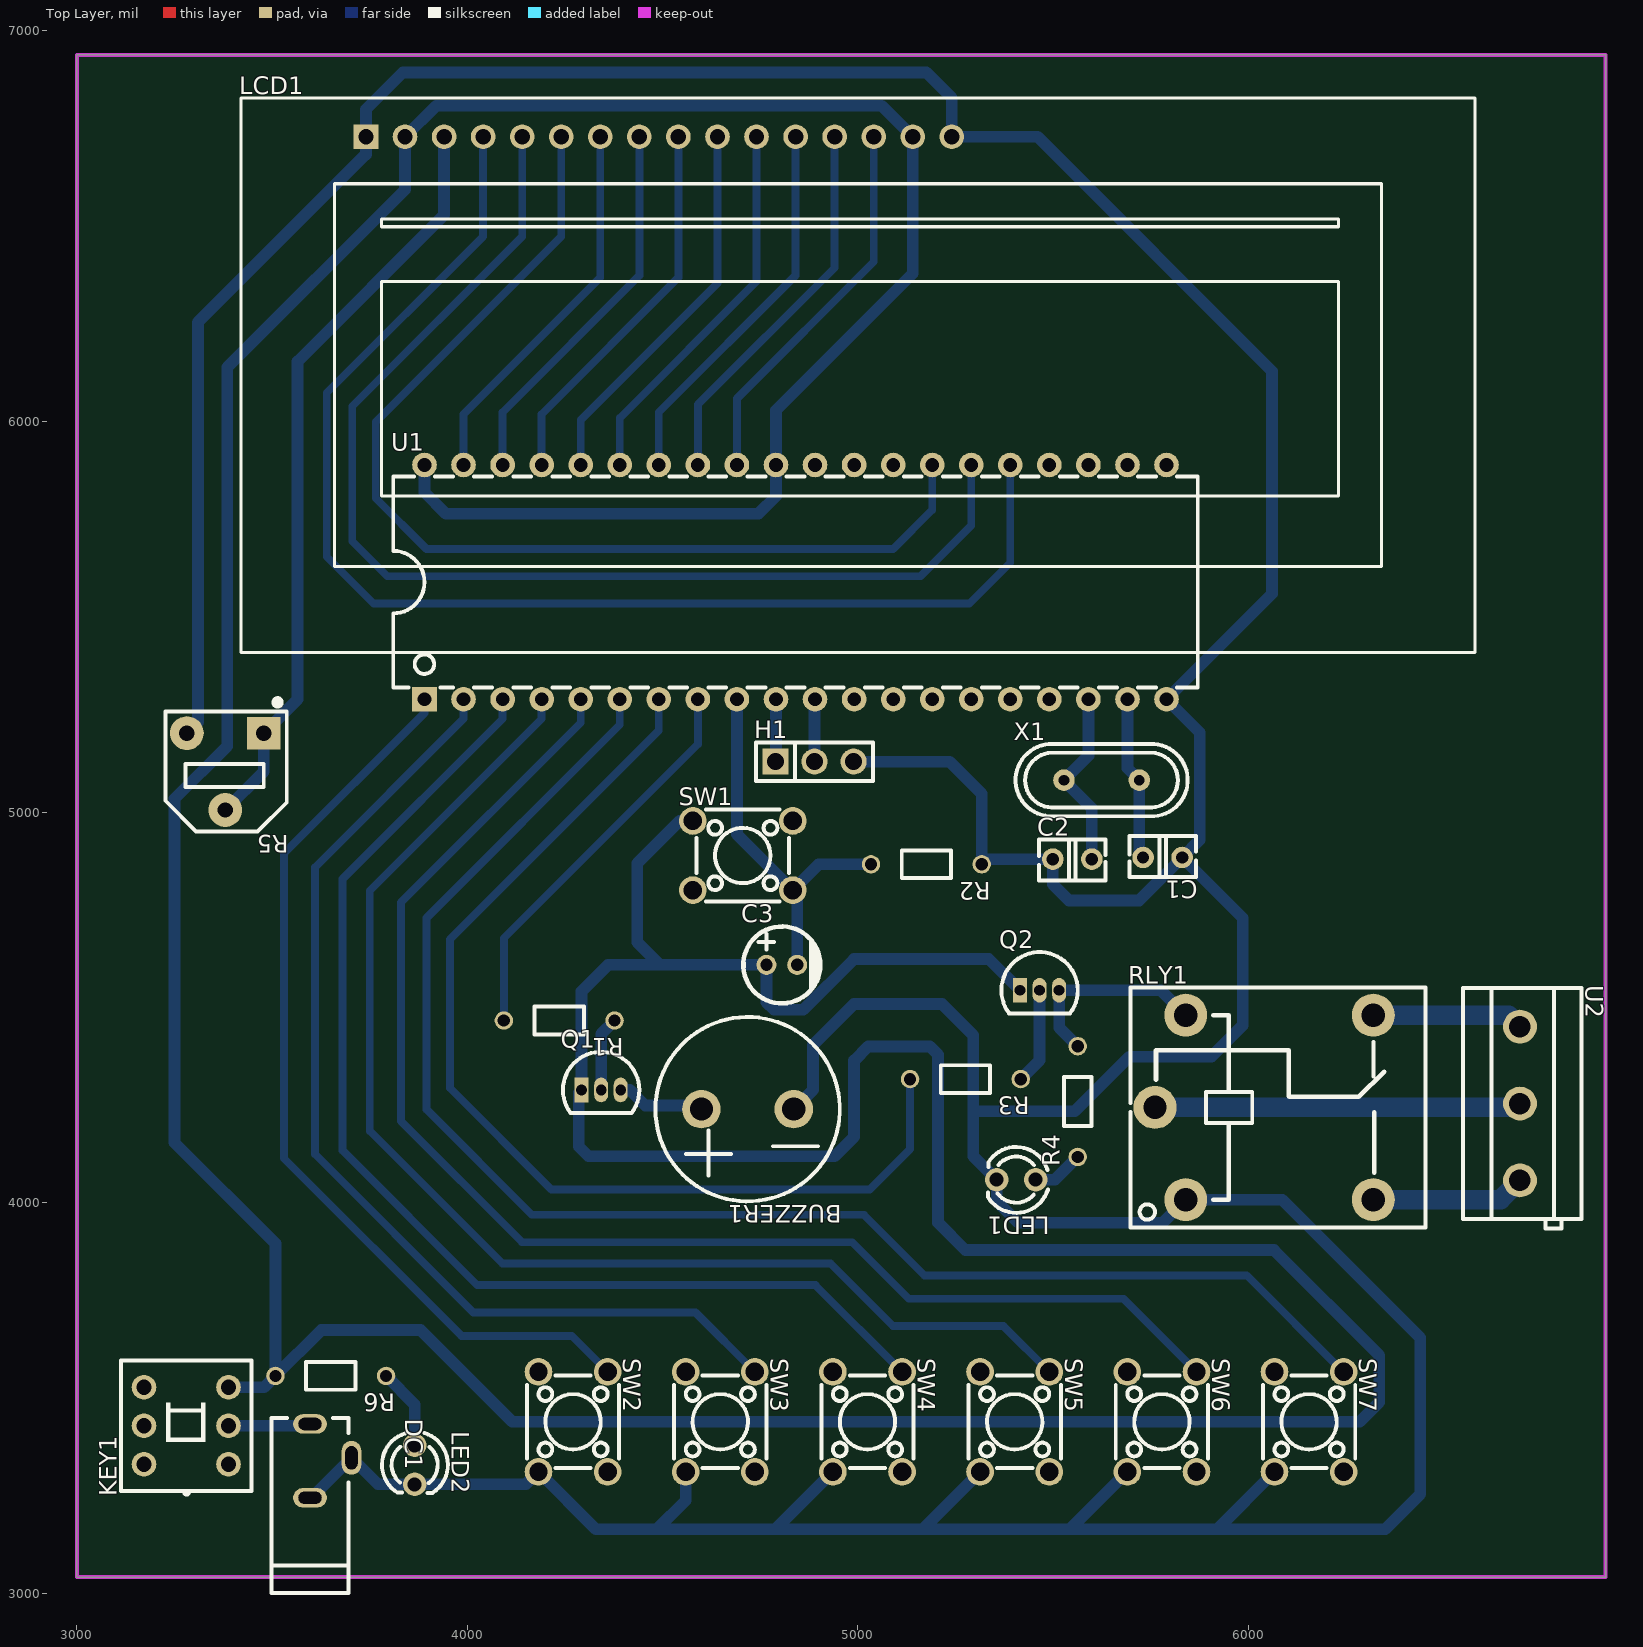
[diagram p0: Top Layer view]
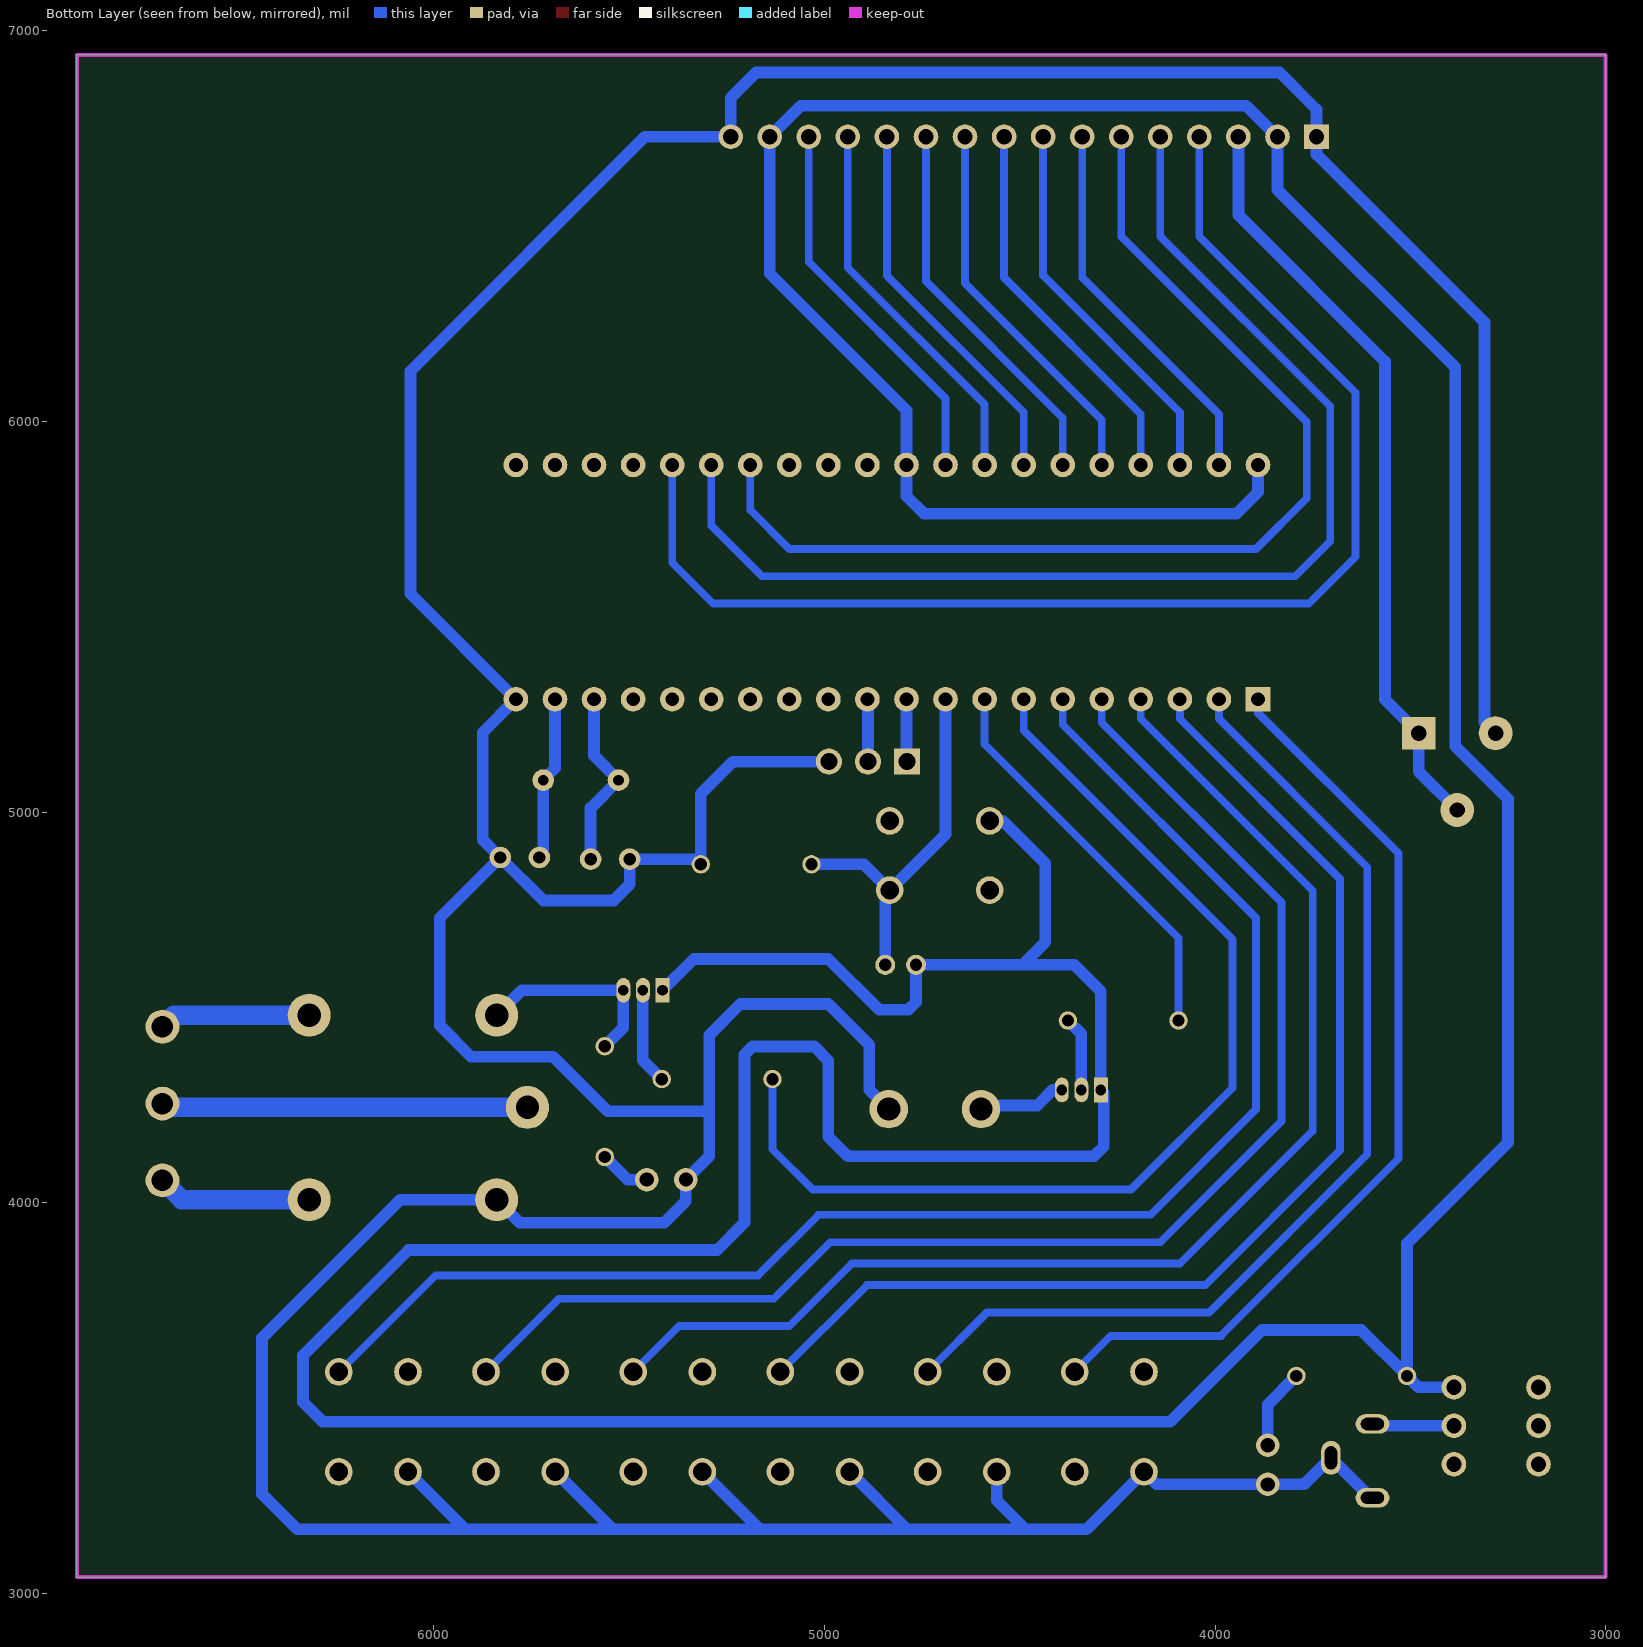
[diagram p1: Bottom Layer view, seen from below]
# Altium PCB MISC50235.pcbdoc
Units mil, origin at the board's own origin, x right, y up, seen from the top; angles counter-clockwise.
Board outline 3914.17 x 3897.64 mil, 2 copper layers (Top Layer, Bottom Layer), stack 62.206 mil thick; 29 components, 48 nets, 137 pads, 0 vias.

## Layer stack, top to bottom
Top Solder Mask Layer: solder mask 0.394, Dk 3.3
Top Layer: signal copper 1.379
Dielectric1: surface 59.449, FR4, Dk 4.5
Bottom Layer: signal copper 1.378
Bottom Solder Mask Layer: solder mask 0.394, Dk 3.3

## Board outline
3000,6938.58 3000,3040.95 6914.17,3040.95 6914.17,6938.58

## Design rules (kind name [scope] priority, off if disabled: settings)
BoardOutlineClearance copperThickness2oz_1 [All] p2 off: genericclearance=7.99 ignorepadtopadclearanceinfootprint=FALSE except(0: Arc-SplitContinuation Track-SplitContinuation SMDPad-SplitContinuation THPad-SplitContinuation Via-SplitContinuation Fill-SplitContinuation Region-SplitContinuation Poly-SplitContinuation Text-SplitContinuation Hole-SplitContinuation; 5.98: Arc-CutoutEdge SMDPad-CutoutEdge THPad-CutoutEdge Via-CutoutEdge Fill-CutoutEdge Region-CutoutEdge Text-CutoutEdge; 6.93: Hole-OutlineEdge Hole-CutoutEdge; 10: Poly-OutlineEdge Poly-CutoutEdge; 11.81: Arc-OutlineEdge Track-OutlineEdge SMDPad-OutlineEdge THPad-OutlineEdge Via-OutlineEdge Fill-OutlineEdge Region-OutlineEdge Text-OutlineEdge Track-CutoutEdge)
BoardOutlineClearance copperThickness1oz_1 [All] p4: genericclearance=4.02 ignorepadtopadclearanceinfootprint=FALSE except(0: Arc-SplitContinuation Track-SplitContinuation SMDPad-SplitContinuation THPad-SplitContinuation Via-SplitContinuation Fill-SplitContinuation Region-SplitContinuation Poly-SplitContinuation Text-SplitContinuation Hole-SplitContinuation; 6: SMDPad-CutoutEdge THPad-CutoutEdge Via-CutoutEdge Fill-CutoutEdge Region-CutoutEdge Text-CutoutEdge; 6.93: Hole-OutlineEdge Hole-CutoutEdge; 10: Poly-OutlineEdge Poly-CutoutEdge; 11.8: Arc-OutlineEdge Track-OutlineEdge SMDPad-OutlineEdge THPad-OutlineEdge Via-OutlineEdge Fill-OutlineEdge Region-OutlineEdge Text-OutlineEdge; 11.81: Arc-CutoutEdge Track-CutoutEdge)
Clearance copperThickness2oz [All] p1 off: gap=7.99 ignorepadtopadclearanceinfootprint=FALSE except(5.98: SMDPad-Track SMDPad-SMDPad THPad-Track SMDPad-THPad THPad-THPad Track-Via SMDPad-Via THPad-Via Via-Via Fill-Track Region-Track Fill-SMDPad Region-SMDPad Fill-THPad Region-THPad Fill-Via Region-Via Fill-Fill Fill-Region Region-Region Arc-Track Arc-SMDPad Arc-THPad Arc-Via Fill-Arc Region-Arc Arc-Arc Text-Track SMDPad-Text Text-THPad Text-Via Fill-Text Region-Text Arc-Text Text-Text; 6.93: Hole-Track Hole-SMDPad Hole-THPad Hole-Via Fill-Hole Region-Hole Hole-Arc Hole-Text; 10: Poly-Track Poly-SMDPad Poly-THPad Poly-Via Poly-Fill Poly-Region Poly-Poly Poly-Arc Poly-Text Poly-Hole)
Clearance copperThickness1oz [All] p3: gap=4.02 ignorepadtopadclearanceinfootprint=FALSE except(5.98: SMDPad-Track SMDPad-SMDPad THPad-Track SMDPad-THPad THPad-THPad Track-Via SMDPad-Via THPad-Via Via-Via Fill-Track Region-Track Fill-SMDPad Region-SMDPad Fill-THPad Region-THPad Fill-Via Region-Via Fill-Fill Fill-Region Region-Region; 6: Arc-Track Arc-SMDPad Arc-THPad Arc-Via Fill-Arc Region-Arc Arc-Arc Text-Track SMDPad-Text Text-THPad Text-Via Fill-Text Region-Text Arc-Text Text-Text; 6.93: Hole-Track Hole-SMDPad Hole-THPad Hole-Via Fill-Hole Region-Hole Hole-Arc Hole-Text; 10: Poly-Track Poly-SMDPad Poly-THPad Poly-Via Poly-Fill Poly-Region Poly-Poly Poly-Arc Poly-Text Poly-Hole)
Creepage creepage [All] p1: checkdistance=0 ignoreinternallayers=TRUE applytopolygonpour=TRUE
DiffPairsRouting differentialPair [All] p1: maxlimit=6 minlimit=6 mostfreqgap=6 toplayer_minwidth=5 toplayer_prefwidth=10 toplayer_maxwidth=100 toplayer_mingap=6 toplayer_prefgap=6 toplayer_maxgap=6 bottomlayer_minwidth=5 bottomlayer_prefwidth=10 bottomlayer_maxwidth=100 bottomlayer_mingap=6 bottomlayer_prefgap=6 bottomlayer_maxgap=6 maxuncoupledlength=10
HoleToHoleClearance otherClearance [All] p1: gap=11.81 allowstackedmicrovias=TRUE
Length netLength [All] p1: minlimit=0 maxlimit=0
MatchedLengths netLengthTolerance [All] p1: tolerance=1000
PasteMaskExpansion pasteMaskExpansion [All] p1: expansion=0
PlaneConnect innerPlane [All] p1: planeconnectstyle=Relief reliefexpansion=20 reliefentries=4 reliefconductorwidth=10 reliefairgap=10
PolygonConnect copperRegion [All] p1: connectstyle=Relief reliefconductorwidth=10 reliefentries=4 polygonreliefangle="90 Angle" airgapwidth=10 via.connectstyle=Relief via.reliefconductorwidth=10 via.reliefentries=4 via.polygonreliefangle="90 Angle" via.airgapwidth=10
RoutingVias viaSize [All] p1: holewidth=12.01 width=24.02 viastyle="Through Hole" minholewidth=11.81 minwidth=19.68 maxholewidth=248.03 maxwidth=393.7
SolderMaskExpansion solderMaskExpansion [IsVia] p1: expansion=-1000 istentingtop=TRUE
SolderMaskExpansion solderMaskExpansion [All] p2: expansion=2 istentingtop=FALSE
Width copperThickness2oz_2 [All] p1 off: maxlimit=100 minlimit=8 preferedwidth=10
Width copperThickness1oz_2 [All] p2: maxlimit=100 minlimit=5 preferedwidth=10

## Components (designator, comment, footprint, x,y, rotation, side; value= is the part's Value field where it differs from the comment)
BUZZER1 "buzzer" BUZ-TH_BD12.0-P6.00-D0.9-RD 4717.32,4239.13 r180 top
C1 "30pF" CAP-TH_L3.8-W2.5-P2.54-D0.50 5780,4883.58 r180 top
C2 "30pF" CAP-TH_L3.8-W2.5-P2.54-D0.50 5548.8,4879.31 r0 top
C3 "10uF" CAP-TH_BD5.0-P2.00-D0.8-FD-10UF50VC110GL 4805,4608.58 r0 top
DC1 "DC-002" DC-IN-TH_DC-3510 3650,3338.58 r270 top
H1 "" HDR-TH_3P-P2.54-V-M 4888.8,5129.04 r0 top
KEY1 "无自锁开关 8.5×8.5 无声" SW-TH_6P-L8.5-W8.5-P2.54 3280,3428.58 r90 top
LCD1 "HS1602A" LCD1602 5000,6118.58 r0 top
LED1 "" LED_TH-3mm 5405,4058.58 r180 top
LED2 "" LED_TH-3mm 3865,3328.58 r270 top
Q1 "" S8550P_TO-92 4342.32,4288.34 r0 top
Q2 "" S8550P_TO-92 5465,4543.58 r0 top
R1 "1kΩ" Res_1/8W 4235,4468.58 r180 top
R2 "10kΩ" Res_1/8W 5175,4868.58 r180 top
R3 "1kΩ" Res_1/8W 5275,4318.58 r180 top
R4 "1kΩ" Res_1/8W 5565,4258.58 r90 top
R5 "10kΩ" RES-ADJ-SMD_RM065-V1 3380,5103.58 r180 top
R6 "1kΩ" Res_1/8W 3650,3558.58 r180 top
RLY1 "SRD-05VDC-SL-C" RELAY-TH_SRD-XXVDC-XL-C 6040,4243.58 r0 top
SW1 "" SW-TH_4P-L6.0-W6.0-P4.50-LS6.5 4705,4888.58 r0 top
SW2 "" SW-TH_4P-L6.0-W6.0-P4.50-LS6.5 4270.47,3438.58 r270 top
SW3 "" SW-TH_4P-L6.0-W6.0-P4.50-LS6.5 4647.38,3438.58 r270 top
SW4 "" SW-TH_4P-L6.0-W6.0-P4.50-LS6.5 5024.28,3438.58 r270 top
SW5 "" SW-TH_4P-L6.0-W6.0-P4.50-LS6.5 5401.19,3438.58 r270 top
SW6 "" SW-TH_4P-L6.0-W6.0-P4.50-LS6.5 5778.09,3438.58 r270 top
SW7 "" SW-TH_4P-L6.0-W6.0-P4.50-LS6.5 6155,3438.58 r270 top
U1 "STC89C52RC-40I-PDIP40" DIP-40_L52.0-W13.7-P2.54-LS15.2-BL 4840,5588.58 r0 top
U2 "KF301-5.0-3P" CONN-TH_3P-P5.00_KF301-5.0-3P 6695,4253.58 r270 top
X1 "11.0592MHz" OSC-TH_L11.1-W4.7-P4.88 5623.8,5081.61 r0 top

## Footprints (in the part's own frame and the unit in brackets; to place one, negate y for a bottom-side part, rotate by r counter-clockwise, add the part's x,y. Pads: shape width x height; smd on the part's side, far side on the other; paste and mask are expansions set on the pad)
BUZ-TH_BD12.0-P6.00-D0.9-RD [mm]
  round 2.5 hole 1.5 paste+0 mask+0.05: 1(-3,0) 2(3,0)
  silkscreen extent -5.99,-5.99 5.99,5.99
CAP-TH_BD5.0-P2.00-D0.8-FD-10UF50VC110GL [mm]
  round 1.3 hole 0.8: 1(-1,0) 2(1,0)
  silkscreen extent -2.5,-2.5 2.5,2.5
CAP-TH_L3.8-W2.5-P2.54-D0.50 [mm]
  round 1.4 hole 0.8 paste+0 mask+0.05: 1(-1.27,0) 2(1.27,0)
  silkscreen extent -2.16,-1.4 2.16,1.27
CONN-TH_3P-P5.00_KF301-5.0-3P [mm]
  round 2.2 hole 1.4: 1(-5,0) 2(0,0) 3(5,0)
  silkscreen extent -7.5,-3.7 8.13,4
DC-IN-TH_DC-3510 [mm]
  oval 1.27x2.2 hole 0.8 slot 1.5 at 90 deg: 1(-2.4,-1.35) 2(2.4,-1.35)
  oval 2.2x1.27 hole 0.8 slot 1.5 at 0 deg: 3(-0.2,1.35)
  silkscreen extent -2.8,-3.85 8.6,1.15
DIP-40_L52.0-W13.7-P2.54-LS15.2-BL [mil]
  rect 63x63 hole 35: 1(-950,-300)
  round 63 hole 35: 2(-850,-300) 3(-750,-300) 4(-650,-300) 5(-550,-300) 6(-450,-300) 7(-350,-300) 8(-250,-300) 9(-150,-300) 10(-50,-300) 11(50,-300) 12(150,-300) 13(250,-300) 14(350,-300) 15(450,-300) 16(550,-300) 17(650,-300) 18(750,-300) 19(850,-300) 20(950,-300) 21(950,300) 22(850,300) 23(750,300) 24(650,300) 25(550,300) 26(450,300) 27(350,300) 28(250,300) 29(150,300) 30(50,300) 31(-50,300) 32(-150,300) 33(-250,300) 34(-350,300) 35(-450,300) 36(-550,300) 37(-650,300) 38(-750,300) 39(-850,300) 40(-950,300)
  silkscreen extent -1030,-270 1030,270
HDR-TH_3P-P2.54-V-M [mm]
  rect 1.7x1.7 hole 1.1: 1(-2.54,0)
  round 1.7 hole 1.1: 2(0,0) 3(2.54,0)
  silkscreen extent -3.81,-1.25 3.81,1.25
LCD1602 [mm]
  rect 1.6x1.6 hole 1: 1(-32,15.5)
  round 1.6 hole 1: 2(-29.46,15.5) 3(-26.92,15.5) 4(-24.38,15.5) 5(-21.84,15.5) 6(-19.3,15.5) 7(-16.76,15.5) 8(-14.22,15.5) 9(-11.68,15.5) 10(-9.14,15.5) 11(-6.6,15.5) 12(-4.06,15.5) 13(-1.52,15.5) 14(1.02,15.5) 15(3.56,15.5) 16(6.1,15.5)
  silkscreen extent -40.13,-18.03 40.13,18.03
LED_TH-3mm [mil]
  round 60 hole 36 paste+0 mask+2: 1(-50,0) 2(50,0)
  silkscreen extent -81,-84 72,85
OSC-TH_L11.1-W4.7-P4.88 [mm]
  round 1.4 hole 0.7: 1(-2.45,0) 2(2.45,0)
  silkscreen extent -5.59,-2.35 5.6,2.35
RELAY-TH_SRD-XXVDC-XL-C [mil]
  round 110 hole 60: 1(-200.79,-236.22) 2(279.52,-236.2) 3(279.53,236.2) 4(-200.79,236.22) 5(-279.53,0)
  silkscreen extent -342,-307 413,307
RES-ADJ-SMD_RM065-V1 [mm]
  rect 2.2x2.1 hole 1 paste+0 mask+0.05: 1(-2.5,-2.5)
  round 2.2 hole 1 paste+0 mask+0.05: 2(0,2.5) 3(2.5,-2.5)
  silkscreen extent -4,-4.7 3.9,3.9
Res_1/8W [mil]
  round 47.2 hole 31.5 paste+0 mask+2: 1(-141.7,2.48) 2(141.7,2.48)
  silkscreen extent -63,-33 63,38
S8550P_TO-92 [mm]
  rect 0.9x1.6 hole 0.7 paste+0 mask+0.051: 1(-1.27,0)
  oval 0.9x1.6 hole 0.7 paste+0 mask+0.051: 2(0,0) 3(1.27,0)
  silkscreen extent -2.48,-1.5 2.48,2.48
SW-TH_4P-L6.0-W6.0-P4.50-LS6.5 [mm]
  round 1.8 hole 1.2: 1(-3.25,2.25) 2(3.25,2.25) 3(-3.25,-2.25) 4(3.25,-2.25)
  silkscreen extent -3,-3 3,3
SW-TH_6P-L8.5-W8.5-P2.54 [mm]
  round 1.6 hole 1: 1(-2.5,-2.75) 2(0,-2.75) 3(2.5,-2.75) 4(-2.5,2.75) 5(0,2.75) 6(2.5,2.75)
  silkscreen extent -4.47,-4.25 4.25,4.25

## Nets (pads, with @x,y where several pads share a name; then routed paths per layer and width w, separated by ;. In a path a pad name is that pad's centre, name@x,y a point inside that pad or via, vN(x,y) a via of type N, cw(c..) or ccw(c..) an arc to the next point about the centre after c; other vN are vias at no path point)
$1N46: Q1.2 R1.1 | length 192
  Bottom Layer w30: Q1.2 4342.32,4431.73 R1.1
$1N48: BUZZER1.2 Q1.3 | length 227.3
  Bottom Layer w30: Q1.3 4415.25,4288.34 4455,4248.58 4589.76,4248.58 BUZZER1.2
$1N50: C3.2 R2.2 SW1.4 U1.9 | length 971.7
  Bottom Layer w30: U1.9 4690,4942.95 SW1.4 ; C3.2 4844.37,4788.58 SW1.4 ; R2.2 4899.05,4866.11 SW1.4
$1N55: Q2.2 R3.1 | length 247.5
  Bottom Layer w30: R3.1 5465,4364.41 Q2.2
$1N57: RLY1.5 U2.2 | length 938.7
  Bottom Layer w50: RLY1.5 6685,4243.58 U2.2
$1N58: RLY1.3 U2.1 | length 387.6
  Bottom Layer w50: RLY1.3 6665.65,4479.78 U2.1
$1N59: RLY1.2 U2.3 | length 395.9
  Bottom Layer w50: RLY1.2 6645.65,4007.38 U2.3
$1N62: LED1.1 R4.1 | length 131.7
  Bottom Layer w30: LED1.1 5504.22,4058.58 R4.1
$1N65: Q2.3 R4.2 RLY1.4 | length 513.6
  Bottom Layer w30: R4.2 5515,4447.81 Q2.3 5775.43,4543.58 RLY1.4
$1N70: DC1.1 KEY1.2 | length 210.4
  Bottom Layer w30: KEY1.2 3592.36,3428.58 DC1.1
$1N73: LCD1.3 R5.1 R5.2 | length 1955.7
  Bottom Layer w30: R5.2 3478.43,5103.58 R5.1 3565,5288.58 3565,6153.58 3940.16,6528.74 LCD1.3
$1N77: LED2.1 R6.1 | length 207.9
  Bottom Layer w30: R6.1 3865,3482.81 LED2.1
GND: BUZZER1.1 C1.1 C2.1 DC1.2 DC1.3 H1.3 LCD1.1 LCD1.16 LED1.2 LED2.2 R2.1 R5.3 RLY1.1 SW2.4 SW3.4 SW4.4 SW5.4 SW6.4 SW7.4 U1.20 | length 15230.3
  Bottom Layer w30: R5.3 3310,5230.43 3310,6253.58 3740.16,6683.74 LCD1.1 3740.16,6798.74 3835,6893.58 5175,6893.58 5240.16,6828.42 LCD1.16 5459.76,6728.82 6060,6128.58 6060,5558.58 U1.20 5875,5203.58 5875,4928.58 C1.1 ; DC1.2 3600.78,3244.09 DC1.3 3771.03,3278.58 LED2.2 4149.84,3278.58 SW2.4 4328.94,3163.58 4485.21,3163.58 ; SW3.4 4558.8,3237.17 4485.21,3163.58 ; BUZZER1.1 4885,4288.7 4885,4403.58 4990,4508.58 5215,4508.58 5295,4428.58 5295,4233.58 ; SW4.4 4788.65,3163.58 ; H1.3 5234.54,5129.04 5316.7,5046.88 R2.1 5329.9,4879.31 C2.1 5498.8,4814.78 5540,4773.58 5720,4773.58 C1.1 ; SW5.4 5165.56,3163.58 ; SW6.4 5542.46,3163.58 ; SW7.4 5919.37,3163.58 ; 4485.21,3163.58 4788.65,3163.58 ; 4788.65,3163.58 5165.56,3163.58 ; 5165.56,3163.58 5542.46,3163.58 ; 5295,4233.58 5555,4233.58 5695,4373.58 5905,4373.58 5985,4453.58 5985,4728.58 C1.1 ; 5295,4233.58 5295,4118.58 LED1.2 5355,4003.58 5410,3948.58 5780.43,3948.58 RLY1.1 6086.22,4007.36 6440,3653.58 6440,3253.58 6350,3163.58 5919.37,3163.58 ; 5542.46,3163.58 5919.37,3163.58
P00: LCD1.7 U1.39 | length 985.3
  Bottom Layer w20: U1.39 3990,6018.58 4340.16,6368.74 LCD1.7
P01: LCD1.8 U1.38 | length 985.3
  Bottom Layer w20: U1.38 4090,6023.58 4440.16,6373.74 LCD1.8
P02: LCD1.9 U1.37 | length 985.3
  Bottom Layer w20: U1.37 4190,6018.58 4540.16,6368.74 LCD1.9
P03: LCD1.10 U1.36 | length 985.3
  Bottom Layer w20: U1.36 4290,6003.58 4640.16,6353.74 LCD1.10
P04: LCD1.11 U1.35 | length 985.3
  Bottom Layer w20: U1.35 4390,6008.58 4740.16,6358.74 LCD1.11
P05: LCD1.12 U1.34 | length 985.3
  Bottom Layer w20: U1.34 4490,6023.58 4840.16,6373.74 LCD1.12
P06: LCD1.13 U1.33 | length 985.3
  Bottom Layer w20: U1.33 4590,6043.58 4940.16,6393.74 LCD1.13
P07: LCD1.14 U1.32 | length 985.3
  Bottom Layer w20: U1.32 4690,6058.58 5040.16,6408.74 LCD1.14
P10: SW2.1 U1.1 | length 2379.8
  Bottom Layer w20: U1.1 3890,5253.58 3530,4893.58 3530,4113.58 3985,3658.58 4267,3658.58 SW2.1
P11: SW3.1 U1.2 | length 2679.1
  Bottom Layer w20: U1.2 3990,5238.58 3610,4858.58 3610,4123.58 4015,3718.58 4583.91,3718.58 SW3.1
P12: SW4.1 U1.3 | length 2992.6
  Bottom Layer w20: U1.3 4090,5238.58 3680,4828.58 3680,4133.58 4025,3788.58 4890.81,3788.58 SW4.1
P13: SW5.1 U1.4 | length 3282.6
  Bottom Layer w20: U1.4 4190,5238.58 3750,4798.58 3750,4183.58 4090,3843.58 4930,3843.58 5090,3683.58 5372.72,3683.58 SW5.1
P14: SW6.1 U1.5 | length 3573.2
  Bottom Layer w20: U1.5 4290,5228.58 3830,4768.58 3830,4208.58 4140,3898.58 4985,3898.58 5130,3753.58 5679.62,3753.58 SW6.1
P15: SW7.1 U1.6 | length 3882
  Bottom Layer w20: U1.6 4390,5223.58 3895,4728.58 3895,4238.58 4165,3968.58 5015,3968.58 5170,3813.58 5995,3813.58 6242.05,3566.53 SW7.1
P16: R3.2 U1.7 | length 2724.6
  Bottom Layer w20: U1.7 4490,5208.58 3955,4673.58 3955,4293.58 4215,4033.58 5030,4033.58 5133.3,4136.88 R3.2
P17: R1.2 U1.8 | length 1028.2
  Bottom Layer w20: R1.2 4093.3,4676.88 4590,5173.58 U1.8
P20: U1.21
P21: U1.22
P22: U1.23
P23: U1.24
P24: LCD1.4 U1.25 | length 3334.2
  Bottom Layer w20: LCD1.4 4040.16,6473.74 3640,6073.58 3640,5653.58 3760,5533.58 5285,5533.58 5390,5638.58 U1.25
P25: LCD1.5 U1.26 | length 3046.6
  Bottom Layer w20: LCD1.5 4140.16,6473.74 3705,6038.58 3705,5693.58 3795,5603.58 5160,5603.58 5290,5733.58 U1.26
P26: LCD1.6 U1.27 | length 2757.3
  Bottom Layer w20: LCD1.6 4240.16,6473.74 3765,5998.58 3765,5803.58 3895,5673.58 5090,5673.58 5190,5773.58 U1.27
P27: U1.28
P30: H1.1 U1.10 | length 160
  Bottom Layer w30: H1.1 4790,5130.24 U1.10
P31: H1.2 U1.11 | length 160
  Bottom Layer w30: H1.2 4888.8,5287.39 U1.11
P32: U1.12
P33: U1.13
P34: U1.14
P35: U1.15
P36: U1.16
P37: U1.17
VCC: C3.1 KEY1.3 LCD1.2 LCD1.15 Q1.1 Q2.1 R6.2 SW1.1 U1.31 U1.40 | length 15295.7
  Bottom Layer w30: KEY1.3 3479.2,3527.01 R6.2 ; U1.40 3890,5818.58 3945,5763.58 4745,5763.58 4790,5808.58 U1.31 4790,6028.58 5140.16,6378.74 LCD1.15 5060.4,6808.58 3919.92,6808.58 LCD1.2 3840.16,6593.74 3385,6138.58 3385,5168.58 3250,5033.58 3250,4153.58 3508.3,3895.28 R6.2 ; SW1.1 4543.58,4977.16 4435,4868.58 4435,4666.24 4492.66,4608.58 ; Q2.1 5335,4623.58 4990,4623.58 4860,4493.58 4785,4493.58 4765.63,4512.95 C3.1 4492.66,4608.58 ; R6.2 3625.78,3673.58 3880,3673.58 4115,3438.58 6285,3438.58 6335,3488.58 6335,3608.58 6065,3878.58 5275,3878.58 5205,3948.58 5205,4378.58 5183.79,4399.8 5026.21,4399.8 4990,4363.58 4990,4168.58 4940,4118.58 4310,4118.58 4285,4143.58 4285,4281.01 Q1.1 4292.32,4540.91 4360,4608.58 4492.66,4608.58
X1: C2.2 U1.18 X1.1 | length 464.8
  Bottom Layer w30: U1.18 5590,5144.25 X1.1 5598.8,5010.16 C2.2
X2: C1.2 U1.19 X1.2 | length 421.6
  Bottom Layer w30: U1.19 5690,5111.86 X1.2 5720.25,4893.33 C1.2
pads on no net: KEY1.1 KEY1.4 KEY1.5 KEY1.6 SW1.2 SW1.3 SW2.2 SW2.3 SW3.2 SW3.3 SW4.2 SW4.3 SW5.2 SW5.3 SW6.2 SW6.3 SW7.2 SW7.3 U1.29 U1.30

## Keep-outs
Board Outline Layer:
  the board outline again, w10